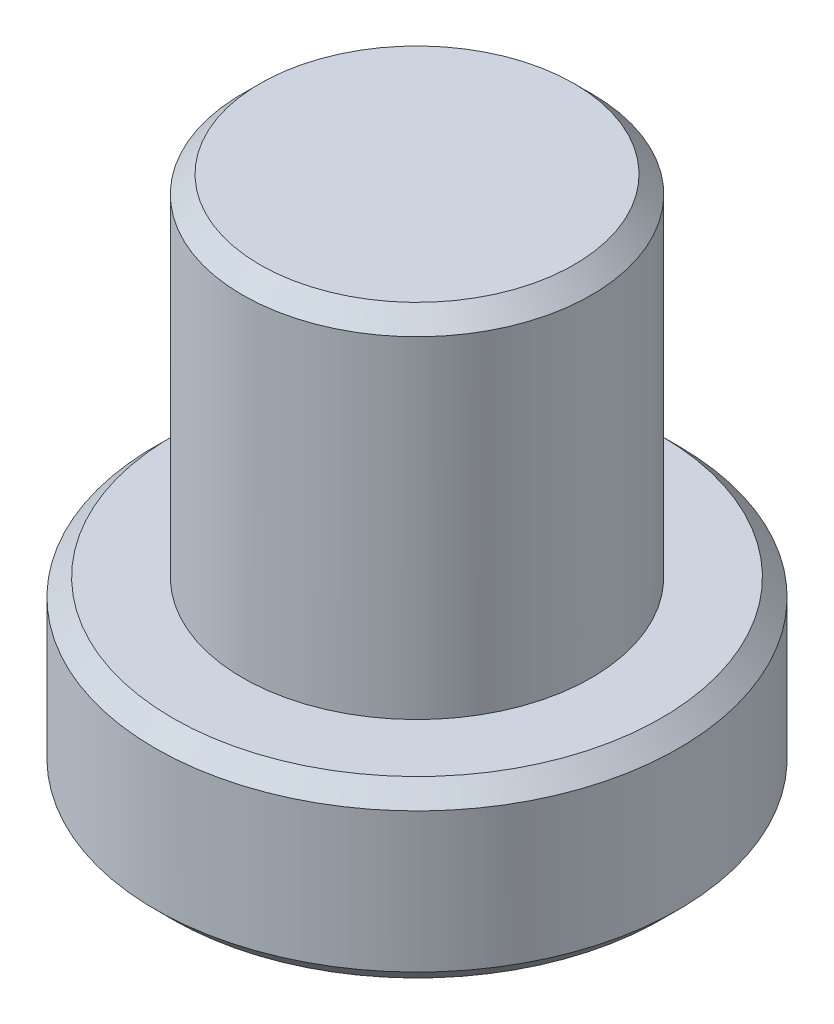
SolidWorks part; units mm, degrees
material "20#"
ref_plane "Front Plane" through (0, 0, 0) normal (0, 0, 1) x (1, 0, 0)
ref_plane "Top Plane" through (0, 0, 0) normal (0, 1, 0) x (1, 0, 0)
ref_plane "Right Plane" through (0, 0, 0) normal (1, 0, 0) x (0, 0, -1)
sketch "Sketch1" plane through (0, 0, 0) normal (1, 0, 0) x (0, 0, -1)
  line L0 (0, 0) -> (0, 15) construction
  line L1 (0, 15) -> (5, 15)
  line L2 (5, 15) -> (5, 5)
  line L3 (5, 5) -> (7.5, 5)
  line L4 (7.5, 5) -> (7.5, 0)
  line L5 (7.5, 0) -> (0, 0)
  line L6 (0, 0) -> (0, 15)
  dimension "D1" = 5
  dimension "D2" = 10
  dimension "D3" = 10
  dimension "D4" = 15
revolve "Revolve1" add sketch "Sketch1" angle 360 about L0
chamfer "Chamfer1" distance 0.5 angle 45 3 edges at (0, 0, -7.5) (0, 5, -7.5) (0, 15, -5)
